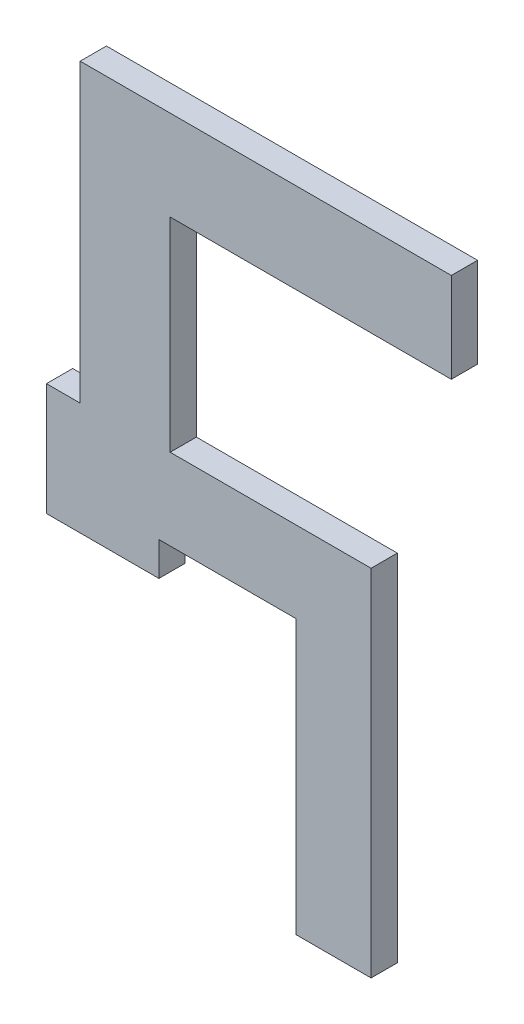
SolidWorks part; units mm, degrees
ref_plane "Front Plane" through (0, 0, 0) normal (0, 0, 1) x (1, 0, 0)
ref_plane "Top Plane" through (0, 0, 0) normal (0, 1, 0) x (1, 0, 0)
ref_plane "Right Plane" through (0, 0, 0) normal (1, 0, 0) x (0, 0, -1)
sketch "Sketch1" plane through (0, 0, 0) normal (0, 0, 1) x (1, 0, 0)
  line L0 (-495, -395) -> (-495, 0)
  line L1 (0, 0) -> (-495, 0)
  line L2 (0, 0) -> (0, -120)
  line L3 (0, -120) -> (-375, -120)
  line L8 (-375, -120) -> (-375, -391.7153)
  line L9 (-495, -395) -> (-540, -395)
  line L10 (-540, -395) -> (-540, -545)
  line L11 (-540, -545) -> (-390, -545)
  line L12 (-390, -545) -> (-390, -500)
  line L13 (-390, -500) -> (-207.0216, -500)
  line L14 (-207.0216, -500) -> (-207.0216, -865)
  line L15 (-207.0216, -865) -> (-107.0216, -865)
  line L16 (-107.0216, -865) -> (-107.0216, -391.7153)
  line L17 (-107.0216, -391.7153) -> (-375, -391.7153)
  dimension "D1" = 120
  dimension "D2" = 120
  dimension "D3" = 100
  dimension "D4" = 545
  dimension "D5" = 150
  dimension "D6" = 45
  dimension "D7" = 45
  dimension "D8" = 150
  dimension "D9" = 320
extrude "Boss-Extrude1" add sketch "Sketch1" along normal blind 35
